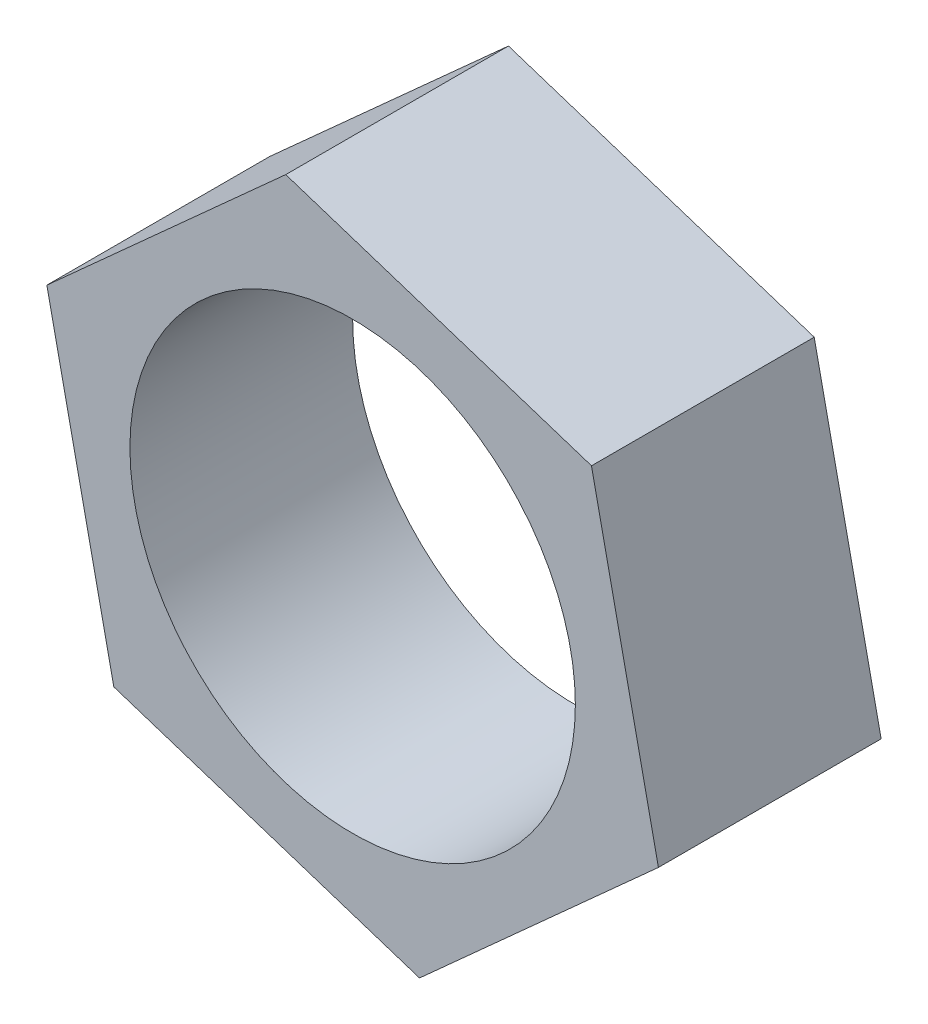
from build123d import *

# Parameters (mm, degrees)
SKETCH1_R           = 10
BOSS_EXTRUDE1_DEPTH = 10


with BuildPart() as part:
    # Sketch1 → Boss-Extrude1 (new body)
    with BuildSketch(Plane.XY):
        Polygon((10.724675699, 9.659951577), (-3.003425616, 14.117817392), (-13.728101315, 4.457865814), (-10.724675699, -9.659951577), (3.003425616, -14.117817392), (13.728101315, -4.457865814), align=None)
        Circle(SKETCH1_R, mode=Mode.SUBTRACT)
    extrude(amount=BOSS_EXTRUDE1_DEPTH)


solid = part.part
